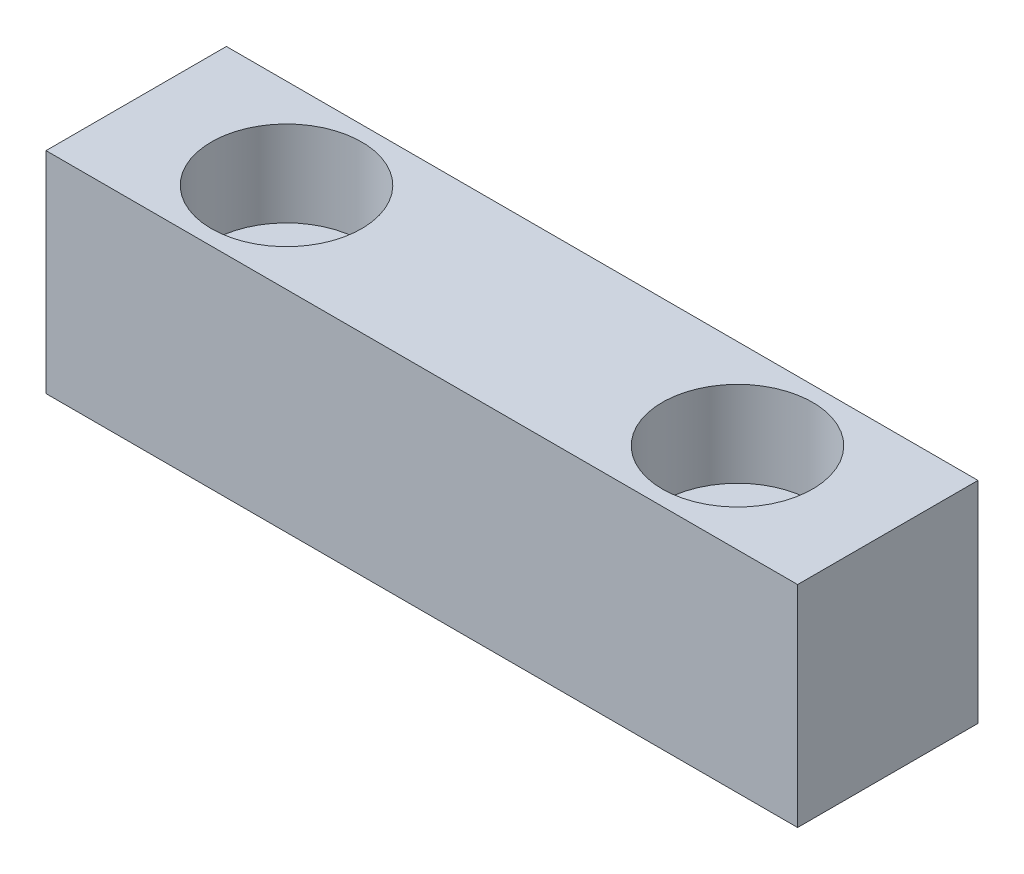
from build123d import *

# Parameters (mm, degrees)
SKETCH1_W                                           = 50
SKETCH1_H                                           = 12
BOSS_EXTRUDE1_DEPTH                                 = 7
HOLE_SIZE_PER_SOCKET_HEAD_CAP_SCREW_TYP_D           = 5.5
HOLE_SIZE_PER_SOCKET_HEAD_CAP_SCREW_TYP_CBORE_D     = 10
HOLE_SIZE_PER_SOCKET_HEAD_CAP_SCREW_TYP_CBORE_DEPTH = 5.7


with BuildPart() as part:
    # Sketch1 → Boss-Extrude1 (new, symmetric)
    with BuildSketch(Plane(origin=(0, 0, 0), x_dir=(1, 0, 0), z_dir=(0, 1, 0))):
        Rectangle(SKETCH1_W, SKETCH1_H)
    extrude(amount=BOSS_EXTRUDE1_DEPTH, both=True)

    # Hole Size (per socket head cap screw type)1 (through all)
    with Locations(Plane(origin=(0, 7, 0), x_dir=(1, 0, 0), z_dir=(0, 1, 0))):
        with Locations((15, 0), (-15, 0)):
            CounterBoreHole(HOLE_SIZE_PER_SOCKET_HEAD_CAP_SCREW_TYP_D / 2, HOLE_SIZE_PER_SOCKET_HEAD_CAP_SCREW_TYP_CBORE_D / 2, HOLE_SIZE_PER_SOCKET_HEAD_CAP_SCREW_TYP_CBORE_DEPTH)


solid = part.part
